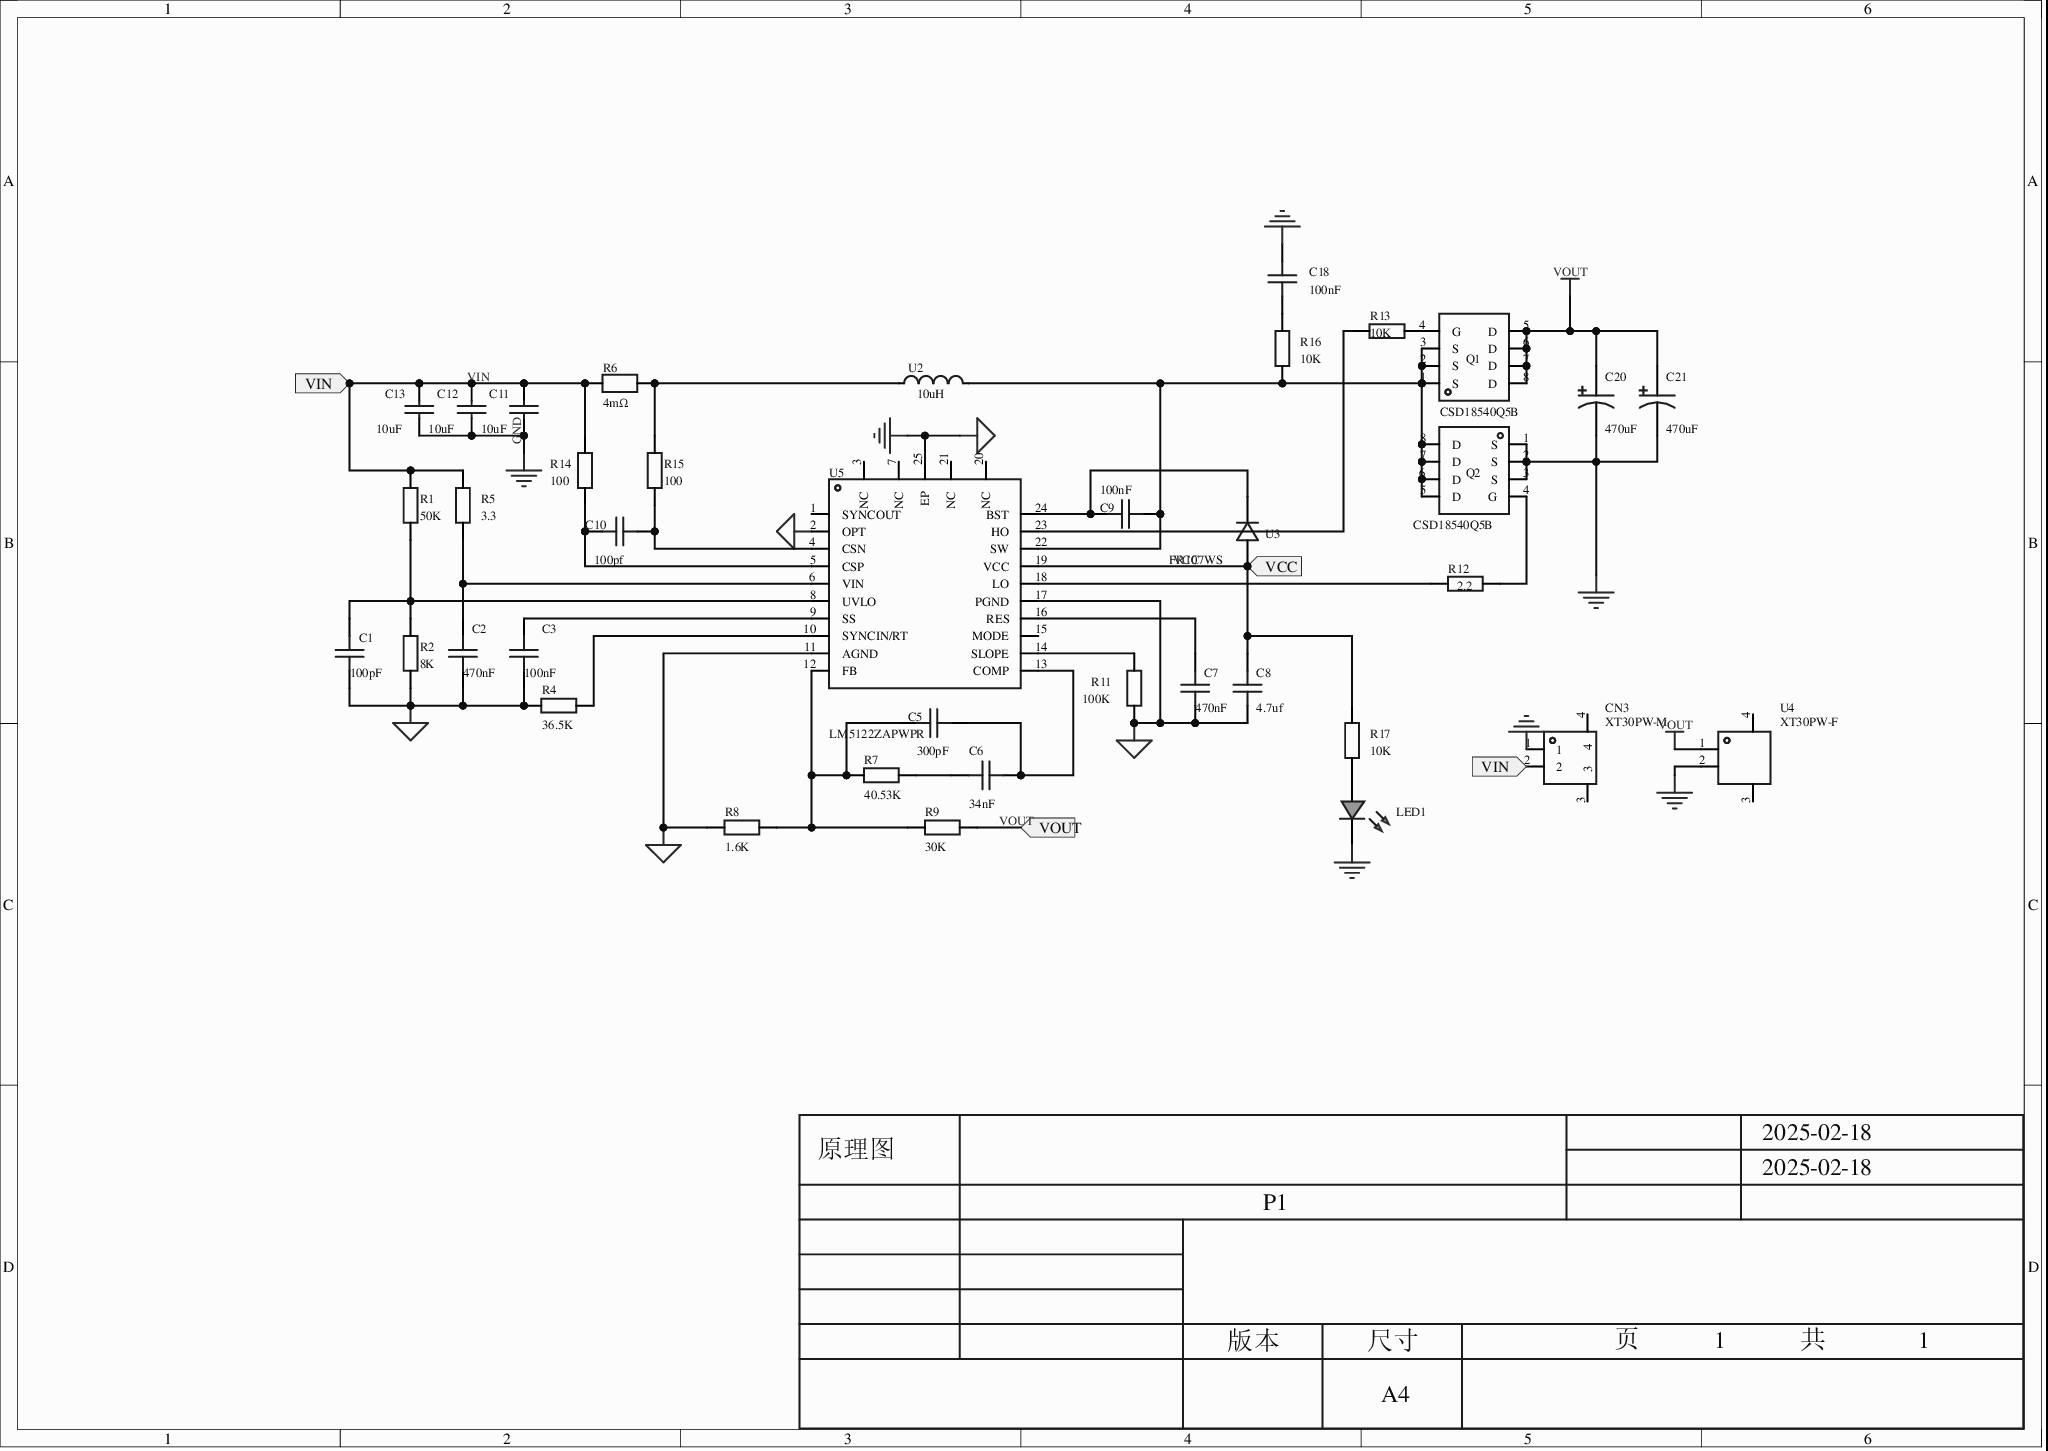
[diagram p0: MISC52028-3.schdoc]
# Altium project MISC52028-2.PrjPcb
1 sheet, 38 parts. Net scope: flat (ports and power ports of the same name join across sheets).
Board file: MISC52028.pcbdoc

## Sheet MISC52028-3.schdoc
size 297 x 210 mm; Version: V1.0; @Project Name: MISC52028; @Page Count: 1; @Update Date: 2025-02-18; @Create Date: 2025-02-18; @Schematic Name: MISC52028; @Page No: 1; @Board Name: MISC52028; @Create Time: 13:14:45; @Update Time: 14:50:02

### Parts
C1  100pF  [C0603]
C2  470nF  [C0603]
C3  100nF  [C0603]
C5  300pF  [C0603]
C6  34nF  [C0603]
C7  470nF  [C0603]
C8  4.7uf  [C0805]
C9  100nF  [C0603]
C10  100pf  [C0603]
C11  10uF  [C1210]
C12  10uF  [C1210]
C13  10uF  [C1210]
C18  100nF  [C0603]
C20  470uF  [CAP-TH_BD16.0-P7.50-D1.2-FD]
C21  470uF  [CAP-TH_BD16.0-P7.50-D1.2-FD]
CN3  XT30PW-M  [CONN-TH_XT30PW-M]
LED1  (no value)  [LED_0805]
Q1  CSD18540Q5B  [VSON-CLIP-8_L5.0-W6.0-P1.27-BL]
Q2  CSD18540Q5B  [VSON-CLIP-8_L5.0-W6.0-P1.27-BL]
R1  50K  [R0603]
R2  8K  [R0603]
R4  36.5K  [R0603]
R5  3.3  [R0805_NEW]
R6  4mΩ  [RES-SMD_L6.4-W3.2-1]
R7  40.53K  [R0603]
R8  1.6K  [R0603]
R9  30K  [R0603]
R11  100K  [R0603]
R12  2.2  [R0603]
R13  10K  [R0603]
R14  100  [R0603]
R15  100  [R0603]
R16  10K  [R0603]
R17  10K  [R0805]
U2  10uH  [IND-SMD_L17.0-W17.0_YSPIA1770-100M]
U3  FR107WS  [SOD-323_L1.6-W1.3-LS2.7-RD]
U4  XT30PW-F  [CONN-TH_XT30PW-F-1]
U5  LM5122ZAPWPR  [HTSSOP-24_L7.8-W4.4-P0.65-LS6.4-BL-EP-3]

### Ports
VCC (in), VIN (in), VOUT (in)

### Nets
AGND: C1.1 C2.1 C3.1 C7.2 C8.2 C11.1 C12.1 C13.1 C18.2 C20.2 C21.2 CN3.1 LED1.1(C) Q2.1(S) Q2.2(S) Q2.3(S) R2.1 R4.1 R8.1 R11.1 U4.2 U5.2(OPT) U5.11(AGND) U5.17(PGND) U5.25(EP)  [also labelled GND]
VOUT: C20.1 C21.1 Q1.5(D) Q1.6(D) Q1.7(D) Q1.8(D) R9.2 U4.1 ; port VOUT
VCC: C8.1 R17.2 U3.2(A) U5.19(VCC) ; port VCC
VIN: C11.2 C12.2 C13.2 CN3.2 R1.2 R5.2 R6.1 R14.2 ; port VIN
NetC1_2: C1.2 R1.1 R2.2 U5.8(UVLO)
NetC2_2: C2.2 R5.1 U5.6(VIN)
NetC3_2: C3.2 U5.9(SS)
NetC5_1: C5.1 R7.1 R8.2 R9.1 U5.12(FB)
NetC5_2: C5.2 C6.2 U5.13(COMP)
NetC6_1: C6.1 R7.2
NetC7_1: C7.1 U5.16(RES)
NetC9_1: C9.1 Q1.1(S) Q1.2(S) Q1.3(S) Q2.5(D) Q2.6(D) Q2.7(D) Q2.8(D) R16.1 U2.2 U5.22(SW)
NetC9_2: C9.2 U3.1(K) U5.24(BST)
NetC10_1: C10.1 R14.1 U5.5(CSP)
NetC10_2: C10.2 R15.1 U5.4(CSN)
NetC18_1: C18.1 R16.2
NetLED1_2: LED1.2(A) R17.1
NetQ1_4: Q1.4(G) R13.2
NetQ2_4: Q2.4(G) R12.2
NetR4_2: R4.2 U5.10(SYNCIN/RT)
NetR6_2: R6.2 R15.2 U2.1
NetR11_2: R11.2 U5.14(SLOPE)
NetR12_1: R12.1 U5.18(LO)
NetR13_1: R13.1 U5.23(HO)

Not connected (* = marked no-connect by the designer): CN3 3* 4*; U4 3* 4*; U5 1(SYNCOUT)* 3(NC)* 7(NC)* 15(MODE)* 20(NC)* 21(NC)*

### Notes on the sheet
- 2025-02-18
- 原理图
- P1
- 版本
- 尺寸
- A4
- 页
- 1
- 共

### Library data of the parts
C1-C3 C5-C7 C9 C10 C18 = CAP_0603: ConvertToPcb: yes; SymbolName: CapAcitance; ModelId: ac125912035d415993ca9572d50418b1; ModelName: C0603_L1.6-W0.8-H0.8; ModelTransform: 62.992,31.496,0,0,0,0,0,0,0; Device: CAP_0603; AddInBom: yes; Supplier Footprint: 0603; FootprintName: C0603
  C1: Value: 100pF
  C2 C7: Value: 470nF
  C3 C9 C18: Value: 100nF
  C5: Value: 300pF
  C6: Value: 34nF
  C10: Value: 100pf
C8 = CAP_0805: ConvertToPcb: yes; SymbolName: CapAcitance; ModelId: 1ba041120af144c991958decab20d241; ModelName: C0805_L2.0-W1.3-H1.3; ModelTransform: 78.74,51.181,0,0,0,0,0,0.0005,0; Value: 4.7uf; Device: CAP_0805; AddInBom: yes; Supplier Footprint: 0805; FootprintName: C0805
C11-C13 = 1210B106K500NT_C116808: 容值:10uF;精度:±10%;额定电压:50V;材质(温度系数):X7R;; Manufacturer: FH(风华); AddInBom: yes; ModelId: 113f675d30df4856af7632edb7ada0df; ModelName: C1210_L3.2-W2.5-H0.9; ModelTransform: 125.984,99.2124,0,0,0,0,0,0,0; Tolerance: ±10%; Voltage Rated: 50V; Temperature Coefficient: X7R; Symbol: 1210B106K500NT; Device: 1210B106K500NT_C116808; Supplier: LCSC; Manufacturer Part: 1210B106K500NT; Value: 10uF; Supplier Part: C116808; JLCPCB Part Class: Extended Part; LCSC Part Name: 10uF ±10% 50V; Supplier Footprint: 1210; Datasheet: https://atta.szlcsc.com/upload/public/pdf/source/20200305/C486355_26A10D38EF8C2A5C37091D0039909270.pdf; ConvertToPcb: yes; FootprintName: C1210
C20 C21 = NXA 100VB470 M 16*25: 容值:470uF;精度:±20%;额定电压:100V;纹波电流:1.65A@100kHz;等效串联电阻(ESR):36mΩ@100kHz;; Manufacturer: SAMYOUNG(韩国三莹); Symbol: NXA-100VB470-M-16*25; AddInBom: yes; ModelId: 37a409aebc9c4ecea75111e7dbe3916f; ModelName: CAP-TH_D16.0-H25.0-P7.50; ModelTransform: 629.88748,629.36,0,0,0,0,0,0,-137.795; Tolerance: ±20%; Voltage Rated: 100V; Pin Spacing: 7.5mm; Lifetime: 10000hrs@105℃; Device: NXA 100VB470 M 16*25; LCSC Part Name: 470uF ±20% 100V; SupplierPart: C350126; ManufacturerPart: NXA 100VB470 M 16*25; Supplier Footprint: 插件,D16xL25mm; JLCPCB Part Class: 扩展库; Datasheet: https://atta.szlcsc.com/upload/public/pdf/source/20190920/C430850_914054AA82C37226ADDF1C96892D647D.pdf; Supplier: LCSC; ConvertToPcb: yes; FootprintName: CAP-TH_BD16.0-P7.50-D1.2-FD; Value: 470uF; Ripple Current: 1.65A@100kHz; Equivalent Series Resistance(ESR): 36mΩ@100kHz; Diameter: 16mm; Height - Seated (Max): 25mm; Operating Temperature: -40℃~+105℃
CN3 = XT30PW-M: 类别:-;类型1:-;; Manufacturer: AMASS(艾迈斯); AddInBom: yes; ModelId: 722652c2597f41cd937322584dc4b29b; ModelTransform: 523.621,549.2115,0,0,0,0,-0.005,-39.568,-78.74; Brand: 艾迈斯; RatedVoltage: DC 500V; InterfaceType: 公头; RatedCurrent: 15A; RecommendedWireGauge: 16/18/20AWG; contact resistance: 1.2mΩ; specifications: 2pin; Symbol: XT30PW-M; Device: XT30PW-M; Supplier: LCSC; Supplier Part: C431092; Manufacturer Part: XT30PW-M; JLCPCB Part Class: Extended Part; LCSC Part Name: AMASS(艾迈斯)航模插头 卧式弯脚 XT30PW-M公头; Supplier Footprint: -; Datasheet: https://atta.szlcsc.com/upload/public/pdf/source/20220222/6A9F22F7850E25B33E1BE430ADF8560B.pdf; ConvertToPcb: yes; FootprintName: CONN-TH_XT30PW-M; ModelName: CONN-TH_XT30PW-M; Model: XT30PW-M; Power: -; Output: -; Input: -; Size: -; Interface: -; Type: 航模插头; Colour: -; MaximumCurrent: -; Type1: -; NumberOfUSBHoles: -; MetalMaterial: -; InsulationMaterial: -; FlameRetardantGrade: -; Belt length: -
LED1 = LED_0805-G: Symbol: LED_G; Convert to PCB: yes; 3D Model: 381ae4d721d6485eaad9d0ca067812b5; 3D Model Transform: 63.9,39.8,31.9,0,0,0,0,0,0; ModelName: LED-0805_G; Device: LED_0805-G; Add into BOM: yes; Supplier Footprint: 0805; FootprintName: LED_0805
Q1 Q2 = CSD18540Q5B: 类型:N沟道;漏源电压(Vdss):60V;连续漏极电流(Id):100A;功率(Pd):3.1W；195W;导通电阻(RDS(on)@Vgs,Id):2.2mΩ@10V,28A;; Manufacturer: TI(德州仪器); AddInBom: yes; ModelId: cf2f3117a71b44c9aa014f616d137869; ModelName: VSON-CLIP-8_L5.0-W6.0-H1.0-P1.27; ModelTransform: 236.22,196.981,0,90,0,0,0,0,0; Type: N沟道; Drain Source Voltage (Vdss): 60V; Continuous Drain Current (Id): 100A; Gate Threshold Voltage (Vgs(th)@Id): 2.3V@250uA; Total Gate Charge (Qg@Vgs): 53nC@10V; Input Capacitance (Ciss@Vds): 4.23nF@30V; Symbol: CSD18540Q5B; Device: CSD18540Q5B; Supplier: LCSC; Supplier Part: C86513; Manufacturer Part: CSD18540Q5B; JLCPCB Part Class: 扩展库; LCSC Part Name: N沟道 耐压:60V 电流:100A; Supplier Footprint: VSON-8(5x6); Datasheet: https://www.ti.com/cn/lit/gpn/csd18540q5b; ConvertToPcb: yes; FootprintName: VSON-CLIP-8_L5.0-W6.0-P1.27-BL; Power Dissipation (Pd): 3.1W；195W; Drain Source On Resistance (RDS(on)@Vgs,Id): 2.2mΩ@10V,28A; Operating Temperature: -55℃~+150℃@(Tj)
R1 R2 R4 R7-R9 R11-R16 = Res_0603: Symbol: 电阻; ConvertToPcb: yes; ModelId: fc143cca1e79419f9cd78b61e9279f08; ModelTransform: 31.8897,63.7794,0,90,0,0,0,0,0; Device: Res_0603; AddInBom: yes; Supplier Footprint: 0603; FootprintName: R0603; ModelName: R0603
  R1: Value: 50K
  R2: Value: 8K
  R4: Value: 36.5K
  R7: Value: 40.53K
  R8: Value: 1.6K
  R9: Value: 30K
  R11: Value: 100K
  R12: Value: 2.2
  R13 R16: Value: 10K
  R14 R15: Value: 100
R5 = Res_0603: Symbol: 电阻; ConvertToPcb: yes; ModelId: fc143cca1e79419f9cd78b61e9279f08; ModelName: R0603; ModelTransform: 31.8897,63.7794,0,90,0,0,0,0,0; Value: 3.3; Device: Res_0603; AddInBom: yes; Supplier Footprint: 0603; FootprintName: R0805_NEW
R6 = PA2512FKF7W0R05E: 电阻类型:-;阻值:50mΩ;精度:±1%;功率:2W;; Manufacturer: YAGEO(国巨); AddInBom: yes; ModelId: 2a92684014bd46c593e4aa7ce823c350; ModelTransform: 251.968,125.984,0,0,0,0,0,0,0; Tolerance: ±1%; Power(Watts): 2W; Temperature Coefficient: ±100ppm/℃; Value: 4mΩ; Device: PA2512FKF7W0R05E; Symbol: PA2512FKF7W0R05E; LCSC Part Name: 50mΩ ±1% 2W; ManufacturerPart: PA2512FKF7W0R05E; Supplier Footprint: 2512; JLCPCB Part Class: 扩展库; Datasheet: https://atta.szlcsc.com/upload/public/pdf/source/20200824/C728352_770FCC25EE85580672A50CB786975A56.pdf; Supplier: LCSC; ConvertToPcb: yes; FootprintName: RES-SMD_L6.4-W3.2-1; ModelName: RES-SMD_L6.4-W3.2-1; Type: -; Operating Temperature Range: -55℃~+170℃
R17 = Res_0805: Symbol: 电阻; ConvertToPcb: yes; ModelId: 37a81e68749a4138bd2dfa6897b24b85; ModelName: R0805_L2.0-W1.3-H0.6; ModelTransform: 78.74,51.181,0,0,0,0,0,-0.0005,0; Device: Res_0805; AddInBom: yes; Supplier Footprint: 0805; Value: 10K; FootprintName: R0805
U2 = CY1770AT125DS-4R7MC: 电感值:4.7uH;精度:±20%;; Manufacturer: Sumida(胜美达); AddInBom: yes; ModelId: 9956a353a7e34d5f995bfac9598dba1a; ModelTransform: 718.5025,669.29,0,0,0,0,-0.001,0,0; Tolerance: ±20%; Value: 10uH; Device: CY1770AT125DS-4R7MC; Symbol: CY1770AT125DS-4R7MC; LCSC Part Name: 4.7uH ±20%; ManufacturerPart: CY1770AT125DS-4R7MC; Supplier Footprint: SMD,17x17.5mm; JLCPCB Part Class: 扩展库; Datasheet: https://atta.szlcsc.com/upload/public/pdf/source/20221031/4071D165700437CEFF1C843D09A46A8A.pdf; Supplier: LCSC; ConvertToPcb: yes; FootprintName: IND-SMD_L17.0-W17.0_YSPIA1770-100M; ModelName: IND-SMD_L17.0-W17.0_YSPIA1770-100M
U3 = FR107WS: Manufacturer: MDD; AddInBom: yes; ModelId: 39bca86493a8419684ee2090e9340edf; ModelTransform: 104.3305,51.181,0,0,0,0,0,0,0; Device: FR107WS; Symbol: FR107WS; LCSC Part Name: FR107WS; SupplierPart: C964087; ManufacturerPart: FR107WS; Supplier Footprint: SOD-323; JLCPCB Part Class: 扩展库; Supplier: LCSC; ConvertToPcb: yes; FootprintName: SOD-323_L1.6-W1.3-LS2.7-RD; ModelName: SOD-323_L1.6-W1.3-LS2.7-RD
U4 = XT30PW-F: 类别:-;类型1:-;; Manufacturer: AMASS(艾迈斯); AddInBom: yes; Brand: 艾迈斯; InterfaceType: 母头; ModelId: f3d657cfcaff41f2be4579c3731b36da; ModelTransform: 523.621,586.613,0,0,0,0,0,-155.511,-78.74; Symbol: XT30PW-F; Device: XT30PW-F; Supplier: LCSC; Supplier Part: C2913282; Manufacturer Part: XT30PW-F; JLCPCB Part Class: 扩展库; LCSC Part Name: AMASS(艾迈斯)电源连接器 母头 XT30PW-F; Supplier Footprint: -; Datasheet: https://atta.szlcsc.com/upload/public/pdf/source/20190916/C428722_DFF78979486FCB0B58C1FC563067EC88.pdf; ConvertToPcb: yes; FootprintName: CONN-TH_XT30PW-F-1; Model: XT30PW-F; Power: -; Output: -; Input: -; Size: -; Interface: -; Type: 航模插头; Colour: -; MaximumCurrent: -; RatedVoltage: -; Type1: -; NumberOfUSBHoles: -; MetalMaterial: -; InsulationMaterial: -; RatedCurrent: -; RecommendedWireGauge: -; FlameRetardantGrade: -; contact resistance: -; Belt length: -; specifications: -; ModelName: CONN-TH_XT30PW-F-1
U5 = LM5122ZAPWPR: 功能类型:升压型；升降压型;输入电压:4.5V~65V;; Manufacturer: TI(德州仪器); AddInBom: yes; Switching Frequency: 875kHz；450kHz; Synchronous Rectification: 是; Number of Outputs: 1; Topology: SEPIC；升压式；反激式; ModelId: bab0d2ddf21a46ff8d53b9eff244127c; ModelTransform: 307.086,251.968,0,0,0,0,0,0,0; Symbol: LM5122ZAPWPR; Device: LM5122ZAPWPR; LCSC Part Name: LM5122ZAPWPR; SupplierPart: C1850331; ManufacturerPart: LM5122ZAPWPR; Supplier Footprint: HTSSOP-24-EP; JLCPCB Part Class: 扩展库; Datasheet: https://www.ti.com/cn/lit/gpn/lm5122za; Supplier: LCSC; ConvertToPcb: yes; Function: 升压型；升降压型; Input Voltage: 4.5V~65V; Operating Temperature: -40℃~+125℃@(TJ); FootprintName: HTSSOP-24_L7.8-W4.4-P0.65-LS6.4-BL-EP-3; ModelName: HTSSOP-24_L7.8-W4.4-P0.65-LS6.4-BL-EP-3